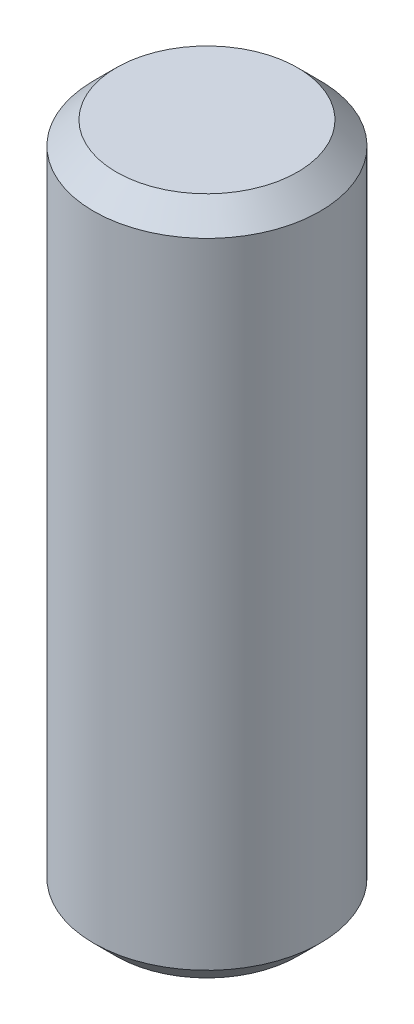
from build123d import *

# Parameters (mm, degrees)
SKETCH_1_R             = 2.5
EXTRUDE_1_DEPTH        = 15
HOLE_WIZARD_M3_1_D     = 2.5
HOLE_WIZARD_M3_1_DEPTH = 7.5
HOLE_WIZARD_M3_1_TIP   = 0.751075774
CHAMFER_1_SIZE         = 0.5


with BuildPart() as part:
    # 草图1 → 凸台-拉伸1 (new body)
    with BuildSketch(Plane(origin=(0, 0, 0), x_dir=(1, 0, 0), z_dir=(0, 1, 0))):
        with Locations(Location((0, 0, 0), (0, 0, 270))):
            Circle(SKETCH_1_R)
    extrude(amount=EXTRUDE_1_DEPTH)

    # M3 螺纹孔1
    with Locations(Plane(origin=(0, 0, 0), x_dir=(-1, 0, 0), z_dir=(0, -1, 0))):
        with Locations((0, 0)):
            Hole(HOLE_WIZARD_M3_1_D / 2, depth=HOLE_WIZARD_M3_1_DEPTH)
            with Locations((0, 0, -(HOLE_WIZARD_M3_1_DEPTH + HOLE_WIZARD_M3_1_TIP / 2))):  # 118° drill point
                Cone(0, HOLE_WIZARD_M3_1_D / 2, HOLE_WIZARD_M3_1_TIP, mode=Mode.SUBTRACT)

    # 倒角1
    chamfer_1_edges = [part.edges().sort_by_distance(p)[0] for p in [
        (0, 0, -2.5),
        (0, 15, -2.5),
    ]]
    chamfer(chamfer_1_edges, length=CHAMFER_1_SIZE)


solid = part.part
